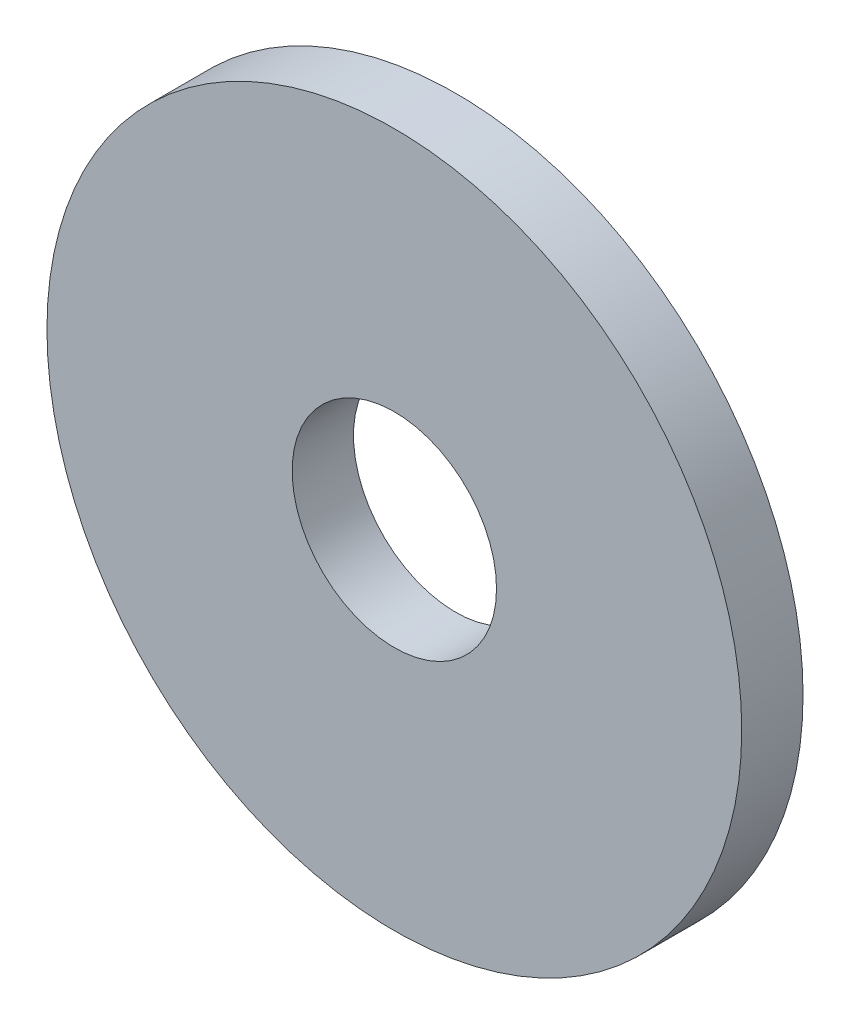
from build123d import *

# Parameters (mm, degrees)
SKETCH1_R           = 85
SKETCH1_R_2         = 25
BOSS_EXTRUDE1_DEPTH = 15


with BuildPart() as part:
    # Sketch1 → Boss-Extrude1 (new body)
    with BuildSketch(Plane.XY):
        Circle(SKETCH1_R)
        Circle(SKETCH1_R_2, mode=Mode.SUBTRACT)
    extrude(amount=BOSS_EXTRUDE1_DEPTH)


solid = part.part
